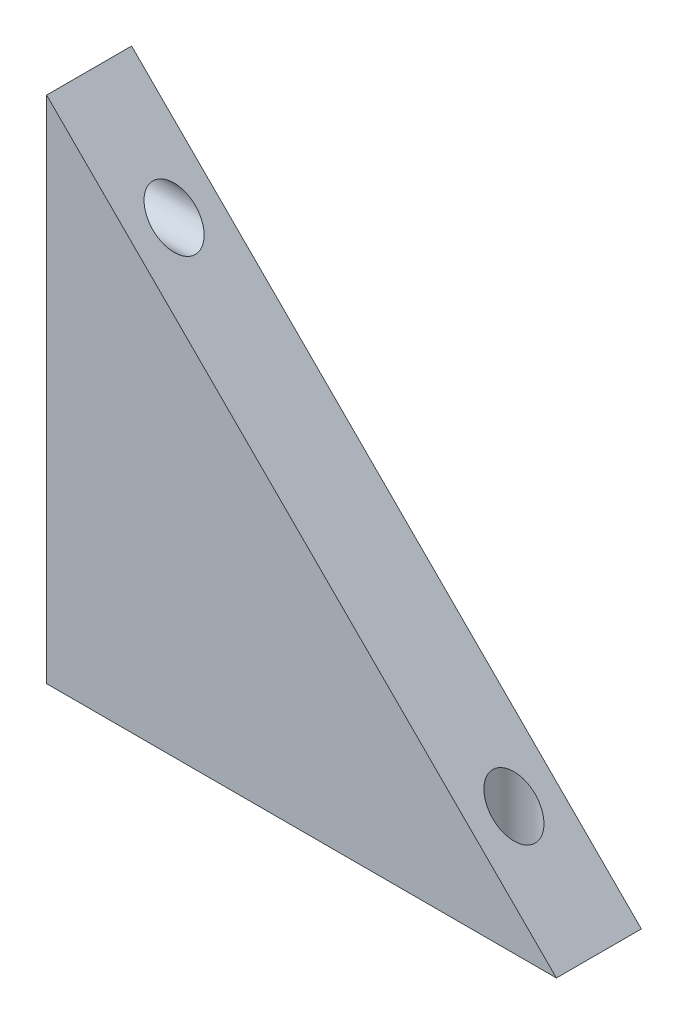
SolidWorks part; units mm, degrees
ref_plane "前视基准面" through (0, 0, 0) normal (0, 0, 1) x (1, 0, 0)
ref_plane "上视基准面" through (0, 0, 0) normal (0, 1, 0) x (1, 0, 0)
ref_plane "右视基准面" through (0, 0, 0) normal (1, 0, 0) x (0, 0, -1)
sketch "草图1" plane through (0, 0, 0) normal (0, 0, 1) x (1, 0, 0)
  line L0 (-30, 30) -> (-30, -30)
  line L1 (-30, -30) -> (30, -30)
  line L2 (-30, 30) -> (30, -30)
  dimension "D1" = 60
  dimension "D2" = 60
  dimension "D3" = 30
extrude "凸台-拉伸1" add sketch "草图1" along normal blind 10
hole_wizard "M6 螺纹孔2" positions "草图2" profile "草图3" tap size "M6" standard "ISO"
sketch "草图2" plane through (0, -30, 0) normal (0, -1, 0) x (-1, 0, 0)
  line L0 (30, -5) -> (-30, -5) construction
  line L1 (30, -10) -> (30, 0) construction
  line L3 (-30, -10) -> (-30, 0) construction
  point P0 (10, -5)
  point P2 (-20, -5)
  dimension "D1" = 20
  dimension "D3" = 30
sketch "草图3" plane through (-10, -30, 5) normal (1, 0, 0) x (0, 0, -1)
  line L0 (0, 0) -> (0, 21.5022)
  line L1 (0, 21.5022) -> (2.5, 20)
  line L2 (2.5, 20) -> (2.5, 0)
  line L5 (2.5, 0) -> (0, 0)
  line L10 (0, 21.5022) -> (-2.5, 20) construction
  line L11 (0, -6.35) -> (0, 107.95) construction
  dimension "螺纹孔钻头直径" = 5
  dimension "螺纹孔钻头深度" = 20
  dimension "导头角度" = 118
cosmetic thread "孔螺蚊线3"
cosmetic thread "孔螺蚊线4"
hole_wizard "M6 螺纹孔1" positions "草图4" profile "草图5" tap size "M6" standard "ISO"
sketch "草图4" plane through (-30, 0, 0) normal (-1, 0, 0) x (0, 0, 1)
  line L0 (5, -30) -> (5, 30) construction
  line L1 (10, -30) -> (0, -30) construction
  line L7 (10, 30) -> (0, 30) construction
  point P2 (5, 20)
  point P4 (5, -10)
  dimension "D1" = 20
  dimension "D2" = 30
sketch "草图5" plane through (-30, 20, 5) normal (0, 1, 0) x (0, 0, 1)
  line L0 (0, 0) -> (0, 21.5022)
  line L1 (0, 21.5022) -> (2.5, 20)
  line L2 (2.5, 20) -> (2.5, 0)
  line L5 (2.5, 0) -> (0, 0)
  line L10 (0, 21.5022) -> (-2.5, 20) construction
  line L11 (0, -6.35) -> (0, 107.95) construction
  dimension "螺纹孔钻头直径" = 5
  dimension "螺纹孔钻头深度" = 20
  dimension "导头角度" = 118
cosmetic thread "孔螺蚊线5"
cosmetic thread "孔螺蚊线6"
